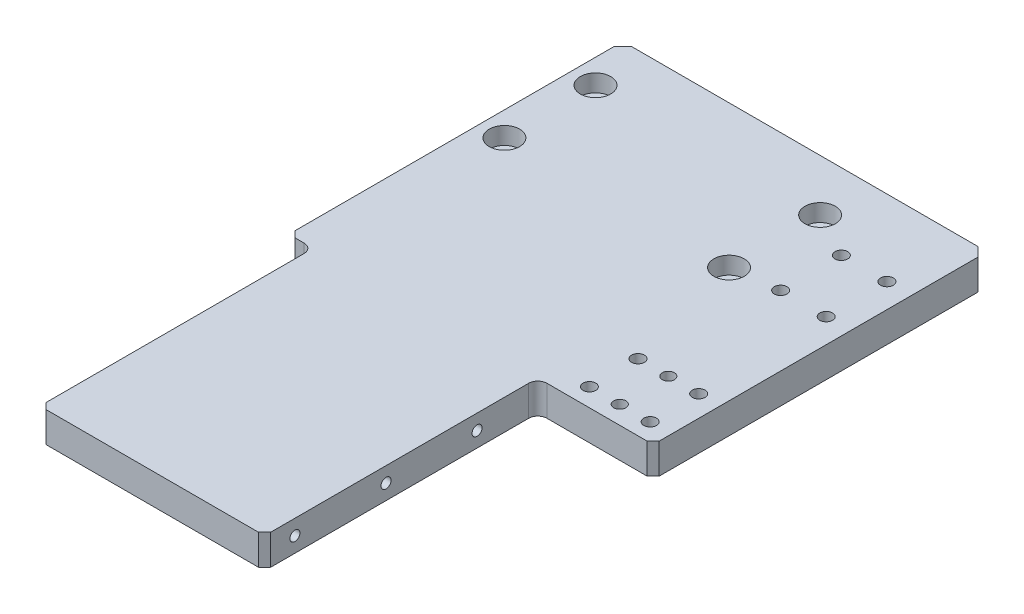
SolidWorks part; units mm, degrees
material "A6061 T6"
ref_plane "前视基准面" through (0, 0, 0) normal (0, 0, 1) x (1, 0, 0)
ref_plane "上视基准面" through (0, 0, 0) normal (0, 1, 0) x (1, 0, 0)
ref_plane "右视基准面" through (0, 0, 0) normal (1, 0, 0) x (0, 0, -1)
sketch "草图1" plane through (0, 0, 0) normal (0, 1, 0) x (1, 0, 0)
  line L1 (-60, 100) -> (60, 100)
  line L2 (-60, 100) -> (-60, -100)
  line L3 (-60, -100) -> (60, -100)
  line L4 (60, 100) -> (60, -100)
  line L5 (-60, 100) -> (60, -100) construction
  line L6 (-60, -100) -> (60, 100) construction
  point P0 (0, 0)
  dimension "D1" = 200
  dimension "D2" = 120
extrude "凸台-拉伸1" add sketch "草图1" along normal blind 10
chamfer "倒角1" distance 3 angle 45 4 edges at (-60, 5, -100) (60, 5, -100) (60, 5, 100) (-60, 5, 100)
hole_wizard "打孔尺寸(%根据)内六角圆柱头螺钉的类型0" positions "草图2" profile "草图3" counterbore size "M5" standard "GB"
sketch "草图2" plane through (0, 10, 0) normal (0, 1, 0) x (1, 0, 0)
  line L0 (-60, 97) -> (-60, -97) construction
  line L1 (57, 100) -> (-57, 100) construction
  line L2 (60, -97) -> (60, 97) construction
  point P16 (-52, 83)
  point P19 (-52, 53)
  point P22 (22, 53)
  point P25 (22, 83)
  dimension "D1" = 30
  dimension "D2" = 8
  dimension "D3" = 17
  dimension "D4" = 38
sketch "草图3" plane through (-52, 10, -83) normal (1, 0, 0) x (0, 0, 1)
  line L0 (0, 0) -> (0, 11.7524)
  line L1 (0, 11.7524) -> (2.75, 10.1)
  line L2 (2.75, 10.1) -> (2.75, 5.7)
  line L3 (2.75, 5.7) -> (5, 5.7)
  line L4 (5, 5.7) -> (5, 0)
  line L5 (5, 0) -> (0, 0)
  line L10 (0, 11.7524) -> (-2.75, 10.1) construction
  line L11 (0, -6.35) -> (0, 107.95) construction
  dimension "孔直径" = 5.5
  dimension "孔深度" = 10.1
  dimension "柱形沉头孔直径" = 10
  dimension "柱形沉头孔深度" = 5.7
  dimension "导头角度" = 118
sketch "草图4" plane through (0, 10, 0) normal (0, 1, 0) x (1, 0, 0)
  line L0 (60, -97) -> (60, 97) construction
  line L1 (60, -10) -> (22, -10)
  line L2 (60, -10) -> (60, -100)
  line L3 (60, -100) -> (22, -100)
  line L4 (22, -10) -> (22, -100)
  line L5 (-57, -100) -> (57, -100) construction
  line L6 (-60, 97) -> (-60, -97) construction
  line L7 (-60, -10) -> (-52, -10)
  line L8 (-60, -10) -> (-60, -100)
  line L9 (-60, -100) -> (-52, -100)
  line L10 (-52, -10) -> (-52, -100)
  dimension "D1" = 74
  dimension "D2" = 90
  dimension "D3" = 8
extrude "切除-拉伸1" cut sketch "草图4" against normal blind 20
chamfer "倒角2" distance 2 angle 45 4 edges at (-60, 5, 10) (-52, 5, 100) (22, 5, 100) (60, 5, 10)
fillet "圆角1" radius 3 2 edges at (-52, 5, 10) (22, 5, 10)
hole_wizard "M4 螺纹孔1" positions "草图5" profile "草图6" tap size "M4" standard "GB"
sketch "草图5" plane through (-52, 0, 0) normal (-1, 0, 0) x (0, 0, 1)
  point P0 (30, 5)
  point P3 (60, 5)
  point P6 (90, 5)
sketch "草图6" plane through (-52, 5, 30) normal (0, 1, 0) x (0, 0, 1)
  line L0 (0, 0) -> (0, 11.0914)
  line L1 (0, 11.0914) -> (1.65, 10.1)
  line L2 (1.65, 10.1) -> (1.65, 0)
  line L5 (1.65, 0) -> (0, 0)
  line L10 (0, 11.0914) -> (-1.65, 10.1) construction
  line L11 (0, -6.35) -> (0, 107.95) construction
  dimension "螺纹孔钻头直径" = 3.3
  dimension "螺纹孔钻头深度" = 10.1
  dimension "导头角度" = 118
cosmetic thread "孔螺蚊线1" parameters "D1"=8, "D2"=4
cosmetic thread "孔螺蚊线2" parameters "D1"=8, "D2"=4
cosmetic thread "孔螺蚊线3" parameters "D1"=8, "D2"=4
hole_wizard "M4 螺纹孔2" positions "草图7" profile "草图8" tap size "M4" standard "GB"
sketch "草图7" plane through (22, 0, 0) normal (1, 0, 0) x (0, 0, -1)
  point P0 (-30, 5)
  point P3 (-60, 5)
  point P6 (-90, 5)
sketch "草图8" plane through (22, 5, 30) normal (0, 1, 0) x (0, 0, -1)
  line L0 (0, 0) -> (0, 11.0914)
  line L1 (0, 11.0914) -> (1.65, 10.1)
  line L2 (1.65, 10.1) -> (1.65, 0)
  line L5 (1.65, 0) -> (0, 0)
  line L10 (0, 11.0914) -> (-1.65, 10.1) construction
  line L11 (0, -6.35) -> (0, 107.95) construction
  dimension "螺纹孔钻头直径" = 3.3
  dimension "螺纹孔钻头深度" = 10.1
  dimension "导头角度" = 118
cosmetic thread "孔螺蚊线4" parameters "D1"=8, "D2"=4
cosmetic thread "孔螺蚊线5" parameters "D1"=8, "D2"=4
cosmetic thread "孔螺蚊线6" parameters "D1"=8, "D2"=4
hole_wizard "大小mm 暗销孔2" positions "草图13" profile "草图14" hole size "Ø4.0" standard "GB"
sketch "草图13" plane through (0, 10, 0) normal (0, 1, 0) x (1, 0, 0)
  point P0 (43, 12)
  point P3 (43, -4)
sketch "草图14" plane through (43, 10, -12) normal (1, 0, 0) x (0, 0, 1)
  line L0 (0, 0) -> (0, 13.6017)
  line L1 (0, 13.6017) -> (2, 12.4)
  line L2 (2, 12.4) -> (2, 0)
  line L5 (2, 0) -> (0, 0)
  line L10 (0, 13.6017) -> (-2, 12.4) construction
  line L11 (0, -6.35) -> (0, 107.95) construction
  dimension "孔直径" = 4
  dimension "孔深度" = 12.4
  dimension "导头角度" = 118
hole_wizard "M5 螺纹孔2" positions "草图15" profile "草图16" tap size "M5" standard "GB"
sketch "草图15" plane through (0, 10, 0) normal (0, 1, 0) x (1, 0, 0)
  point P0 (53, -4)
  point P3 (33, -4)
  point P6 (53, 12)
  point P9 (33, 12)
sketch "草图16" plane through (53, 10, 4) normal (1, 0, 0) x (0, 0, 1)
  line L0 (0, 0) -> (0, 13.6618)
  line L1 (0, 13.6618) -> (2.1, 12.4)
  line L2 (2.1, 12.4) -> (2.1, 0)
  line L5 (2.1, 0) -> (0, 0)
  line L10 (0, 13.6618) -> (-2.1, 12.4) construction
  line L11 (0, -6.35) -> (0, 107.95) construction
  dimension "螺纹孔钻头直径" = 4.2
  dimension "螺纹孔钻头深度" = 12.4
  dimension "导头角度" = 118
cosmetic thread "孔螺蚊线11"
cosmetic thread "孔螺蚊线12"
cosmetic thread "孔螺蚊线13"
cosmetic thread "孔螺蚊线14"
hole_wizard "M5 螺纹孔3" positions "草图17" profile "草图18" tap size "M5" standard "GB"
sketch "草图17" plane through (0, 10, 0) normal (0, 1, 0) x (1, 0, 0)
  point P0 (52, 55)
  point P3 (37, 55)
  point P6 (52, 75)
  point P9 (37, 75)
sketch "草图18" plane through (52, 10, -55) normal (1, 0, 0) x (0, 0, 1)
  line L0 (0, 0) -> (0, 13.6618)
  line L1 (0, 13.6618) -> (2.1, 12.4)
  line L2 (2.1, 12.4) -> (2.1, 0)
  line L5 (2.1, 0) -> (0, 0)
  line L10 (0, 13.6618) -> (-2.1, 12.4) construction
  line L11 (0, -6.35) -> (0, 107.95) construction
  dimension "螺纹孔钻头直径" = 4.2
  dimension "螺纹孔钻头深度" = 12.4
  dimension "导头角度" = 118
cosmetic thread "孔螺蚊线15"
cosmetic thread "孔螺蚊线16"
cosmetic thread "孔螺蚊线17"
cosmetic thread "孔螺蚊线18"
